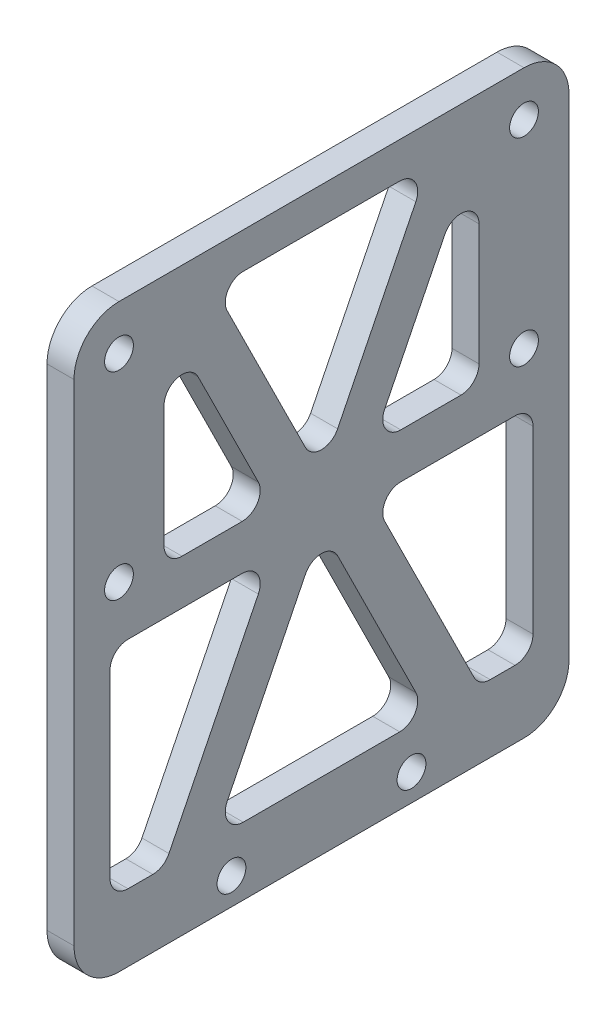
from build123d import *

# Parameters (mm, degrees)
SKETCH_2_W          = 55
SKETCH_2_H          = 64.5
EXTRUDE_1_DEPTH     = 3
SKETCH_3_R          = 1.6
CUT_EXTRUDE_1_DEPTH = 3
FILLET_1_R          = 5
CUT_EXTRUDE_2_DEPTH = 3
FILLET_2_R          = 2


with BuildPart() as part:
    # 草图2 → 凸台-拉伸1 (new body)
    with BuildSketch(Plane(origin=(0, 0, 0), x_dir=(0, 0, -1), z_dir=(1, 0, 0))):
        with Locations((27.5, 32.25)):
            Rectangle(SKETCH_2_W, SKETCH_2_H)
    extrude(amount=EXTRUDE_1_DEPTH)

    # 草图3 → 切除-拉伸1 (cut)
    with BuildSketch(Plane.ZY):
        with Locations((-5, 59.5)):
            Circle(SKETCH_3_R)
        with Locations((-5, 37.5)):
            Circle(SKETCH_3_R)
        with Locations((-50, 59.5)):
            Circle(SKETCH_3_R)
        with Locations((-50, 37.5)):
            Circle(SKETCH_3_R)
        with Locations((-37.5, 3)):
            Circle(SKETCH_3_R)
        with Locations((-17.5, 3)):
            Circle(SKETCH_3_R)
    extrude(amount=-CUT_EXTRUDE_1_DEPTH, mode=Mode.SUBTRACT)

    # 圆角1
    fillet_1_edges = [part.edges().sort_by_distance(p)[0] for p in [
        (1.5, 64.5, 0),
        (1.5, 64.5, -55),
        (1.5, 0, -55),
        (1.5, 0, 0),
    ]]
    fillet(fillet_1_edges, radius=FILLET_1_R)

    # 草图4 → 切除-拉伸2 (cut)
    with BuildSketch(Plane.ZY):
        Polygon((-39.417495765, 60.5), (-27.5, 36.5), (-15.582504235, 60.5), align=None)
        Polygon((-45, 60.5), (-45, 36.5), (-33.082504235, 36.5), align=None)
        Polygon((-21.917495765, 36.5), (-10, 60.5), (-10, 36.5), align=None)
        Polygon((-10, 31.5), (-21.917495765, 31.5), (-10, 7.5), (-4, 7.5), (-4, 31.5), align=None)
        Polygon((-39.417495765, 7.5), (-27.5, 31.5), (-15.582504235, 7.5), align=None)
        Polygon((-45, 31.5), (-33.082504235, 31.5), (-45, 7.5), (-51, 7.5), (-51, 31.5), align=None)
    extrude(amount=-CUT_EXTRUDE_2_DEPTH, mode=Mode.SUBTRACT)

    # 圆角2
    fillet_2_edges = [part.edges().sort_by_distance(p)[0] for p in [
        (1.5, 60.5, -45),
        (1.5, 36.5, -33.082504235),
        (1.5, 36.5, -45),
        (1.5, 60.5, -39.417495765),
        (1.5, 60.5, -15.582504235),
        (1.5, 36.5, -27.5),
        (1.5, 31.5, -27.5),
        (1.5, 7.5, -15.582504235),
        (1.5, 7.5, -39.417495765),
        (1.5, 31.5, -4),
        (1.5, 7.5, -4),
        (1.5, 7.5, -10),
        (1.5, 31.5, -21.917495765),
        (1.5, 7.5, -51),
        (1.5, 31.5, -51),
        (1.5, 31.5, -33.082504235),
        (1.5, 7.5, -45),
        (1.5, 36.5, -10),
        (1.5, 36.5, -21.917495765),
        (1.5, 60.5, -10),
    ]]
    fillet(fillet_2_edges, radius=FILLET_2_R)


solid = part.part
